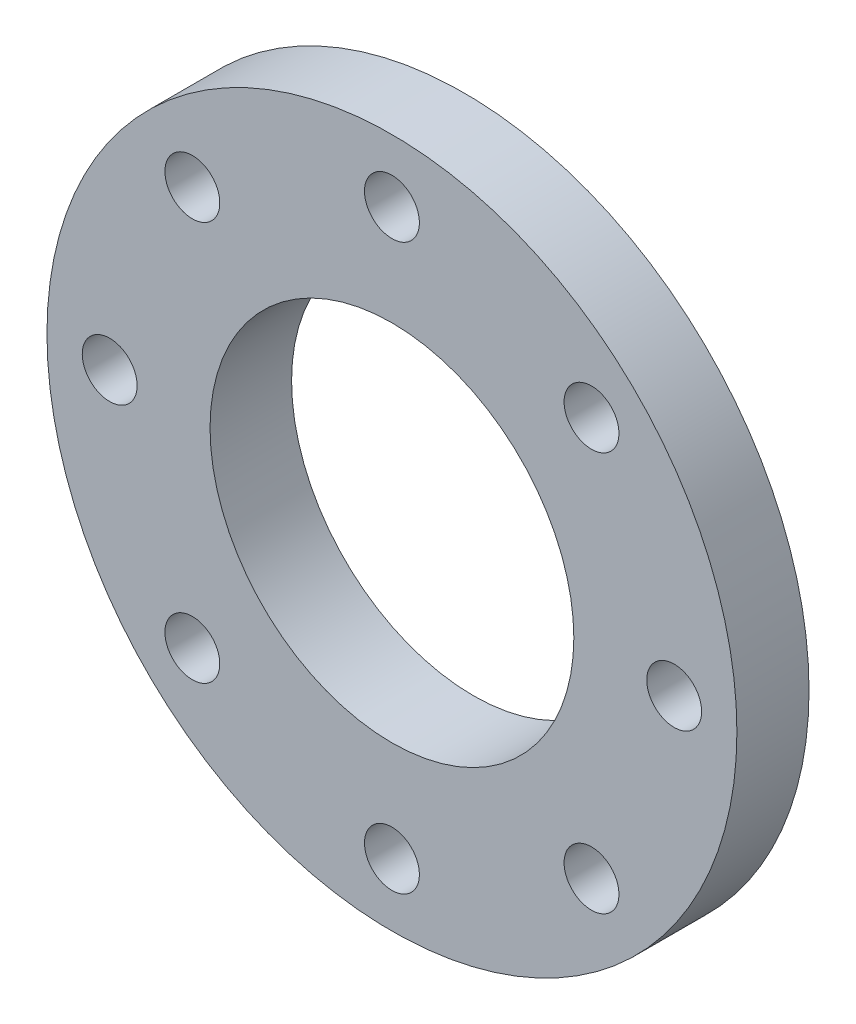
from build123d import *

# Parameters (mm, degrees)
SKETCH1_R               = 110
SKETCH1_R_2             = 8.75
BOSS_EXTRUDE1_DEPTH     = 26
CUT_EXTRUDE2_DEPTH      = 158.721273137
CUT_EXTRUDE2_DEPTH_BACK = 158.721273137
SKETCH3_R               = 58


with BuildPart() as part:
    # Sketch1 → Boss-Extrude1 (new body)
    with BuildSketch(Plane.XY):
        with Locations(Location((0, 0, 0), (0, 0, 180))):
            Circle(SKETCH1_R)
        with Locations(Location((0, 90, 0), (0, 0, 180))):
            Circle(SKETCH1_R_2, mode=Mode.SUBTRACT)
        with Locations(Location((63.639610307, 63.639610307, 0), (0, 0, 180))):
            Circle(SKETCH1_R_2, mode=Mode.SUBTRACT)
        with Locations(Location((90, 0, 0), (0, 0, 180))):
            Circle(SKETCH1_R_2, mode=Mode.SUBTRACT)
        with Locations(Location((63.639610307, -63.639610307, 0), (0, 0, 180))):
            Circle(SKETCH1_R_2, mode=Mode.SUBTRACT)
        with Locations(Location((0, -90, 0), (0, 0, 180))):
            Circle(SKETCH1_R_2, mode=Mode.SUBTRACT)
        with Locations(Location((-63.639610307, -63.639610307, 0), (0, 0, 180))):
            Circle(SKETCH1_R_2, mode=Mode.SUBTRACT)
        with Locations(Location((-90, 0, 0), (0, 0, 180))):
            Circle(SKETCH1_R_2, mode=Mode.SUBTRACT)
        with Locations(Location((-63.639610307, 63.639610307, 0), (0, 0, 180))):
            Circle(SKETCH1_R_2, mode=Mode.SUBTRACT)
    extrude(amount=BOSS_EXTRUDE1_DEPTH)

    # Sketch3 → Cut-Extrude2 (cut, two sides: drawn at the far end of the back side and taken through both)
    with BuildSketch(Plane.XY.offset(26).offset(-CUT_EXTRUDE2_DEPTH_BACK)):
        Circle(SKETCH3_R)
    extrude(amount=CUT_EXTRUDE2_DEPTH + CUT_EXTRUDE2_DEPTH_BACK, mode=Mode.SUBTRACT)

    # Sketch4 → Cut-Revolve1 (revolve, cut)
    with BuildSketch(Plane(origin=(0, 0, 0), x_dir=(1, 0, 0), z_dir=(0, 1, 0)), mode=Mode.PRIVATE) as cut_revolve1_sk:
        Polygon((79, 0), (81, -3), (110, -3), (110, 0), align=None)
    revolve(cut_revolve1_sk.sketch.rotate(Axis((0, 0, 0), (0, 0, 1)), 180), axis=Axis((0, 0, 0), (0, 0, 1)), mode=Mode.SUBTRACT)


solid = part.part
